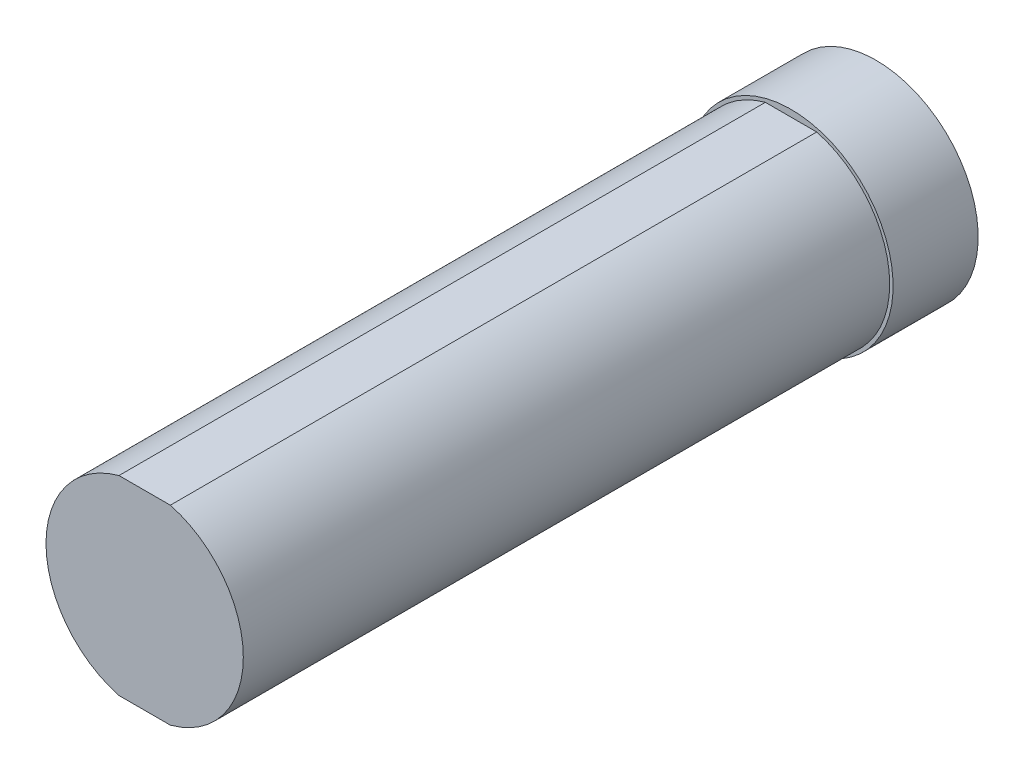
SolidWorks part; units mm, degrees
ref_plane "Front Plane" through (0, 0, 0) normal (0, 0, 1) x (1, 0, 0)
ref_plane "Top Plane" through (0, 0, 0) normal (0, 1, 0) x (1, 0, 0)
ref_plane "Right Plane" through (0, 0, 0) normal (1, 0, 0) x (0, 0, -1)
sketch "Sketch1" plane through (0, 0, 0) normal (0, 0, 1) x (1, 0, 0)
  circle A0 centre (0, 0) radius 29
  dimension "D1" = 58
extrude "Boss-Extrude1" add sketch "Sketch1" along normal blind 190
sketch "Sketch2" plane through (0, 0, 0) normal (0, 0, -1) x (-1, 0, 0)
  circle A0 centre (0, 0) radius 30
  dimension "D1" = 60
extrude "Boss-Extrude2" add sketch "Sketch2" along normal blind 25
sketch "Sketch4" plane through (0, 0, 190) normal (0, 0, 1) x (1, 0, 0)
  line L1 (42.0994, 28) -> (-42.0994, 28)
  line L2 (42.0994, 28) -> (42.0994, -28)
  line L3 (42.0994, -28) -> (-42.0994, -28)
  line L4 (-42.0994, 28) -> (-42.0994, -28)
  line L5 (42.0994, 28) -> (-42.0994, -28) construction
  line L6 (42.0994, -28) -> (-42.0994, 28) construction
  point P0 (0, 0)
  dimension "D1" = 56
extrude "Cut-Extrude1" cut sketch "Sketch4" against normal up to surface (190 mm away) flip side to cut up to face at (29, 0, 0)
sketch "Sketch5" plane through (0, 0, -25) normal (0, 0, -1) x (-1, 0, 0)
  circle A0 centre (0, 0) radius 24
  dimension "D1" = 48
extrude "Cut-Extrude2" cut sketch "Sketch5" against normal blind 22
sketch "Sketch6" plane through (0, 0, -3) normal (0, 0, -1) x (-1, 0, 0)
  circle A0 centre (0, 0) radius 24.1
  dimension "D1" = 48.2
extrude "Cut-Extrude3" cut sketch "Sketch6" against normal blind 3
sketch "Sketch7" plane through (0, 0, 0) normal (0, 0, -1) x (-1, 0, 0)
  circle A0 centre (0, 0) radius 18
  dimension "D1" = 36
extrude "Cut-Extrude4" cut sketch "Sketch7" against normal blind 180
sketch "Sketch8" plane through (0, 0, 0) normal (0, 1, 0) x (1, 0, 0)
  line L0 (7.5498, -190) -> (-7.5498, -190) construction
  circle A0 centre (0, -55) radius 5
  circle A1 centre (0, -130) radius 7.5
  dimension "D1" = 15
  dimension "D2" = 10
  dimension "D3" = 60
  dimension "D4" = 135
extrude "Cut-Extrude5" cut sketch "Sketch8" against normal blind 180
chamfer "Chamfer1" distance 1 angle 45 1 edges at (-24, 0, -25)
